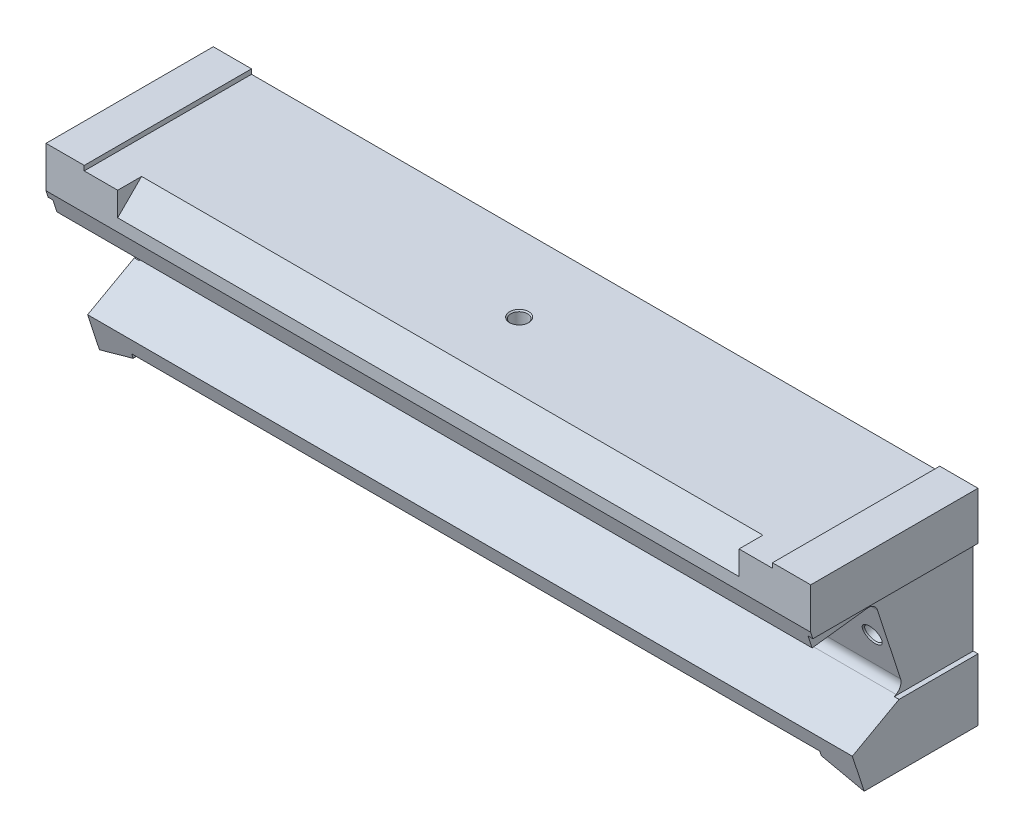
SolidWorks part; units mm, degrees
material "ZG270-500"
ref_plane "Front Plane" through (0, 0, 0) normal (0, 0, 1) x (1, 0, 0)
ref_plane "Top Plane" through (0, 0, 0) normal (0, 1, 0) x (1, 0, 0)
ref_plane "Right Plane" through (0, 0, 0) normal (1, 0, 0) x (0, 0, -1)
sketch "Sketch1" plane through (0, 0, 0) normal (1, 0, 0) x (0, 0, -1)
  line L0 (0, 0) -> (-119.1, 0)
  line L1 (-119.1, 0) -> (-131.4295, 37.9462)
  line L2 (-175, 172.0425) -> (-175, 215)
  line L3 (-175, 215) -> (0, 215)
  line L4 (0, 215) -> (0, 165)
  line L5 (0, 165) -> (-51.7936, 165)
  line L6 (-51.7936, 165) -> (-19.3016, 65)
  line L7 (-19.3016, 65) -> (0, 65)
  line L8 (0, 65) -> (0, 0)
  line L9 (-168.5115, 152.073) -> (-102.7885, 160.1428)
  line L10 (-102.7885, 160.1428) -> (-73.5151, 70.0486)
  line L11 (-73.5151, 70.0486) -> (-131.4295, 37.9462)
  line L12 (-150, 95) -> (-26.3036, 135.1914) construction
  line L13 (-168.5115, 152.073) -> (-175, 172.0425)
  point P17 (-88.1518, 115.0957)
  dimension "D1" = 175
  dimension "D2" = 215
  dimension "D3" = 50
  dimension "D4" = 115
  dimension "D5" = 65
  dimension "D6" = 120
  dimension "D7" = 119.1
  dimension "D8" = 11
  dimension "D9" = 11
  dimension "D10" = 50
  dimension "D11" = 25
  dimension "D12" = 120
  dimension "D13" = 18
extrude "Boss-Extrude1" add sketch "Sketch1" along normal mid plane 800
sketch "Sketch3" plane through (0, 0, 0) normal (0, 0, 1) x (1, 0, 0)
  line L0 (400, 215) -> (-400, 215) construction
  line L1 (360, 210) -> (-360, 210)
  line L2 (360, 210) -> (360, 220)
  line L3 (360, 220) -> (-360, 220)
  line L4 (-360, 210) -> (-360, 220)
  line L5 (360, 210) -> (-360, 220) construction
  line L6 (360, 220) -> (-360, 210) construction
  line L7 (-400, 215) -> (-400, 172.0425) construction
  point P0 (0, 215)
  dimension "D1" = 5
  dimension "D2" = 40
extrude "Cut-Extrude1" cut sketch "Sketch3" along normal through all
sketch "Sketch4" plane through (0, 0, 0) normal (1, 0, 0) x (0, 0, -1)
  line L0 (-175, 215) -> (-175, 185)
  line L1 (-175, 215) -> (-175, 172.0425) construction
  line L2 (-175, 185) -> (-145, 215)
  line L3 (0, 215) -> (-175, 215) construction
  line L4 (-145, 215) -> (-175, 215)
  dimension "D1" = 45
  dimension "D2" = 30
extrude "Cut-Extrude2" cut sketch "Sketch4" against normal mid plane 650
sketch "Sketch6" plane through (0, 0, 0) normal (0, 0, -1) x (-1, 0, 0)
  line L0 (-400, 0) -> (-360, 14.5588)
  line L1 (360, 14.5588) -> (360, 19.5588)
  line L2 (-400, 0) -> (-400, 65) construction
  line L4 (0, 0) -> (0, 24.4492) construction
  line L5 (400, 0) -> (360, 14.5588)
  line L6 (400, 0) -> (-400, 0)
  line L7 (360, 19.5588) -> (-360, 19.5588)
  line L8 (-360, 19.5588) -> (-360, 14.5588)
  dimension "D1" = 40
  dimension "D3" = 5
  dimension "D2" = 70
extrude "Cut-Extrude3" cut sketch "Sketch6" against normal blind 650
sketch "Sketch7" plane through (0, 0, 0) normal (0, 0, 1) x (1, 0, 0)
  line L0 (-400, 37.9462) -> (-400, 0) construction
  line L1 (-405, 165) -> (-395, 165)
  line L2 (-405, 165) -> (-405, 65)
  line L3 (-405, 65) -> (-395, 65)
  line L4 (-395, 165) -> (-395, 65)
  line L5 (-405, 165) -> (-395, 65) construction
  line L6 (-405, 65) -> (-395, 165) construction
  line L7 (-400, 215) -> (-400, 172.0425) construction
  line L8 (-360, 215) -> (-400, 215) construction
  point P0 (-400, 115)
  dimension "D1" = 5
  dimension "D2" = 50
  dimension "D3" = 65
extrude "Cut-Extrude4" cut sketch "Sketch7" along normal blind 650
mirror "Mirror1" about plane through (0, 0, 0) normal (1, 0, 0) of "Cut-Extrude4"
sketch "Sketch8" plane through (0, 0, 0) normal (0, 0, -1) x (-1, 0, 0)
  line L0 (0, 0) -> (0, 260.3656) construction
  line L1 (-400, 165) -> (400, 165) construction
  line L2 (20, 65) -> (-20, 65)
  line L3 (20, 65) -> (20, 165)
  line L4 (20, 165) -> (-20, 165)
  line L5 (-20, 65) -> (-20, 165)
  line L6 (20, 65) -> (-20, 165) construction
  line L7 (20, 165) -> (-20, 65) construction
  line L8 (-395, 65) -> (395, 65) construction
  line L9 (190, 115) -> (-190, 115) construction
  line L10 (-395, 165) -> (395, 165) construction
  line L11 (-170, 65) -> (-210, 65)
  line L12 (-170, 65) -> (-170, 165)
  line L13 (-170, 165) -> (-210, 165)
  line L14 (-210, 65) -> (-210, 165)
  line L15 (-170, 65) -> (-210, 165) construction
  line L16 (-170, 165) -> (-210, 65) construction
  line L18 (210, 65) -> (170, 65)
  line L19 (210, 65) -> (210, 165)
  line L20 (210, 165) -> (170, 165)
  line L21 (170, 65) -> (170, 165)
  line L22 (210, 65) -> (170, 165) construction
  line L23 (210, 165) -> (170, 65) construction
  line L24 (-360, 65) -> (-395, 65)
  line L25 (-360, 65) -> (-360, 165)
  line L26 (-360, 165) -> (-395, 165)
  line L27 (-395, 65) -> (-395, 165)
  line L28 (-360, 65) -> (-395, 165) construction
  line L29 (-360, 165) -> (-395, 65) construction
  line L30 (395, 65) -> (360, 65)
  line L31 (395, 65) -> (395, 165)
  line L32 (395, 165) -> (360, 165)
  line L33 (360, 65) -> (360, 165)
  line L34 (395, 65) -> (360, 165) construction
  line L35 (395, 165) -> (360, 65) construction
  point P3 (0, 115)
  point P15 (0, 115)
  point P25 (-377.5, 115)
  point P30 (377.5, 115)
  dimension "D1" = 40
  dimension "D2" = 40
  dimension "D3" = 40
  dimension "D4" = 150
  dimension "D5" = 150
  dimension "D6" = 35
  dimension "D7" = 150
  dimension "D8" = 35
extrude "Boss-Extrude2" add sketch "Sketch8" against normal up to surface (19.3016 mm away)
sketch "Sketch9" plane through (0, 210, 0) normal (0, 1, 0) x (1, 0, 0)
  line L0 (0, 0) -> (0, -80) construction
  line L1 (-360, 0) -> (360, 0) construction
  dimension "D1" = 80
hole_wizard "M20 Tapped Hole1" positions "3DSketch1" profile "Sketch10" tap size "M20" standard "GB"
sketch3d "3DSketch1"
  point P0 (0, 210, 80)
sketch "Sketch10" plane through (0, 210, 80) normal (1, 0, 0) x (0, 0, 1)
  line L0 (0, 0) -> (0, 50.2575)
  line L1 (0, 50.2575) -> (8.75, 45)
  line L2 (8.75, 45) -> (8.75, 1.275)
  line L3 (8.75, 1.275) -> (10.025, 0)
  line L5 (10.025, 0) -> (0, 0)
  line L6 (-8.75, 1.275) -> (-10.025, 0) construction
  line L10 (0, 50.2575) -> (-8.75, 45) construction
  line L11 (0, -6.35) -> (0, 107.95) construction
  dimension "螺纹孔钻头直径" = 17.5
  dimension "螺纹孔钻头深度" = 45
  dimension "近端锥形沉头孔直径" = 20.05
  dimension "近端锥形沉头孔角度" = 90
  dimension "导头角度" = 118
cosmetic thread "hole cosmetic thread 1" parameters "D1"=40, "D2"=20
sketch "Sketch11" plane through (0, -14.9165, 45.9083) normal (0, -0.309, 0.9511) x (1, 0, 0)
  line L0 (377.5, 136.7029) -> (-377.5, 136.7029) construction
  line L3 (0, 0) -> (0, 136.7029) construction
  point P3 (0, 136.7029)
  dimension "D1" = 755
hole_wizard "M20 Tapped Hole2" positions "3DSketch2" profile "Sketch12" tap size "M20" standard "GB"
sketch3d "3DSketch2"
  point P0 (-377.5, 115.0957, 88.1518)
  point P3 (0, 115.0957, 88.1518)
  point P6 (377.5, 115.0957, 88.1518)
sketch "Sketch12" plane through (-377.5, 115.0957, 88.1518) normal (1, 0, 0) x (0, -0.9511, -0.309)
  line L0 (0, 0) -> (0, 45.2575)
  line L1 (0, 45.2575) -> (8.75, 40)
  line L2 (8.75, 40) -> (8.75, 1.275)
  line L3 (8.75, 1.275) -> (10.025, 0)
  line L5 (10.025, 0) -> (0, 0)
  line L6 (-8.75, 1.275) -> (-10.025, 0) construction
  line L10 (0, 45.2575) -> (-8.75, 40) construction
  line L11 (0, -6.35) -> (0, 107.95) construction
  dimension "螺纹孔钻头直径" = 17.5
  dimension "螺纹孔钻头深度" = 40
  dimension "近端锥形沉头孔直径" = 20.05
  dimension "近端锥形沉头孔角度" = 90
  dimension "导头角度" = 118
cosmetic thread "hole cosmetic thread 2" parameters "D1"=40, "D2"=20
cosmetic thread "hole cosmetic thread 3" parameters "D1"=40, "D2"=20
cosmetic thread "hole cosmetic thread 4" parameters "D1"=40, "D2"=20
fillet "Fillet1" radius 10 2 edges at (0, 70.0486, 73.5151) (0, 160.1428, 102.7885)
